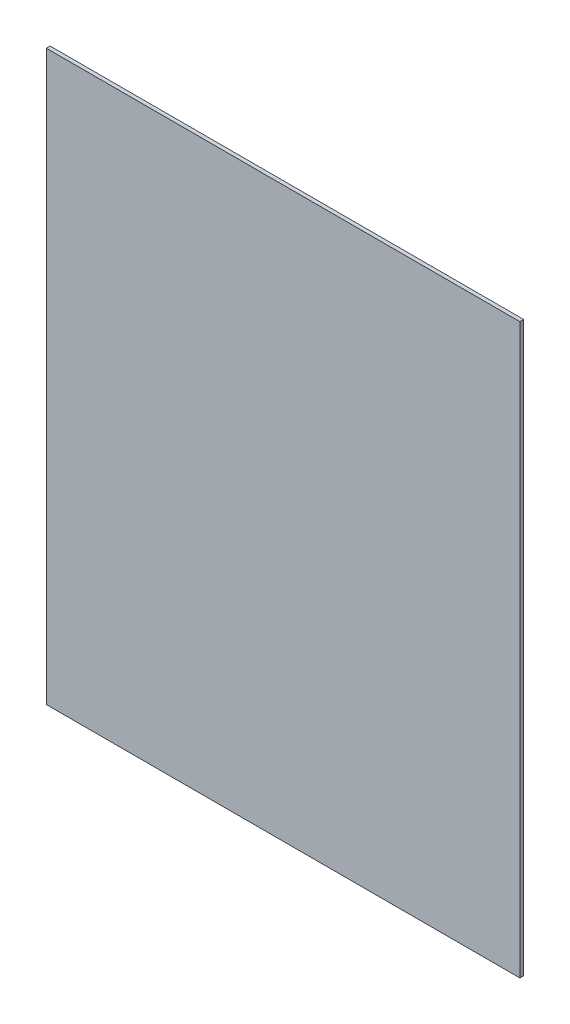
from build123d import *

# Parameters (mm, degrees)
SKETCH1_W           = 250
SKETCH1_H           = 300
BOSS_EXTRUDE1_DEPTH = 2


with BuildPart() as part:
    # Sketch1 → Boss-Extrude1 (new body)
    with BuildSketch(Plane.XY):
        with Locations((125, 150)):
            Rectangle(SKETCH1_W, SKETCH1_H)
    extrude(amount=BOSS_EXTRUDE1_DEPTH)


solid = part.part
